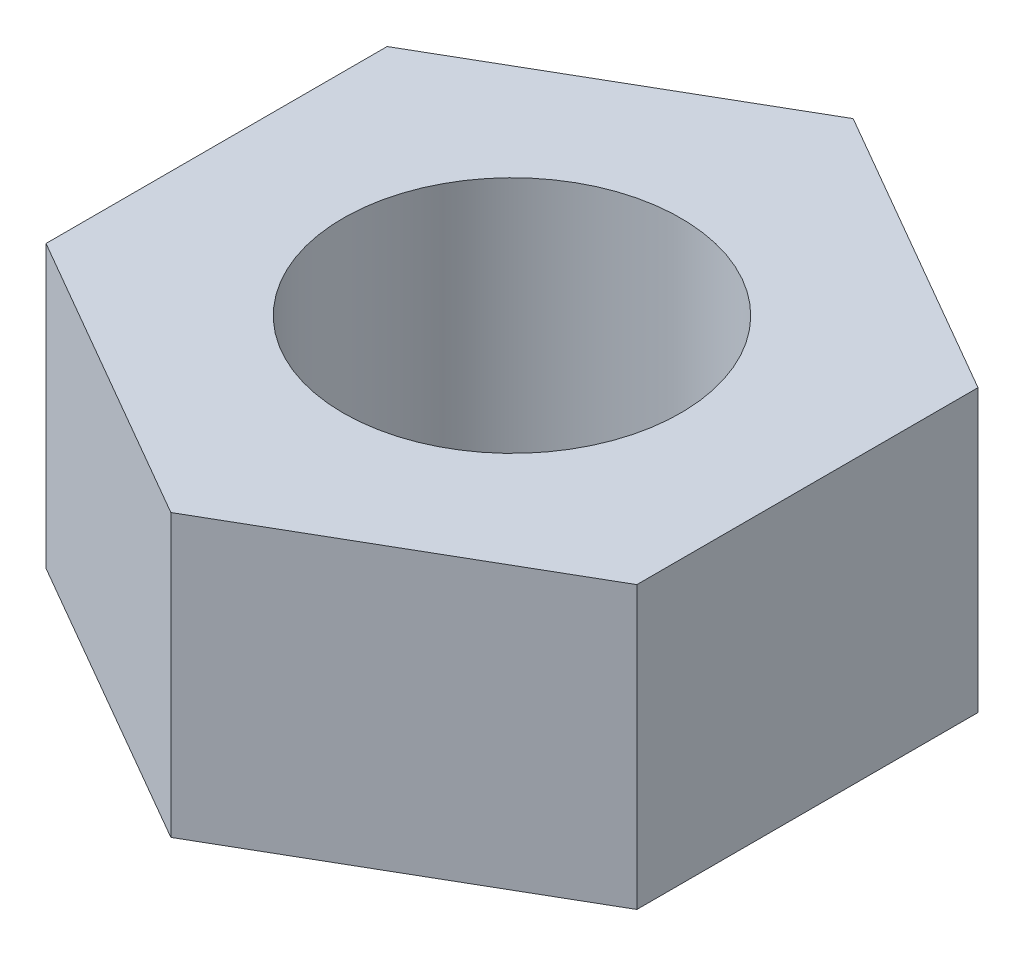
SolidWorks part; units mm, degrees
ref_plane "前视基准面" through (0, 0, 0) normal (0, 0, 1) x (1, 0, 0)
ref_plane "上视基准面" through (0, 0, 0) normal (0, 1, 0) x (1, 0, 0)
ref_plane "右视基准面" through (0, 0, 0) normal (1, 0, 0) x (0, 0, -1)
sketch "草图1" plane through (0, 0, 0) normal (0, 1, 0) x (1, 0, 0)
  line L0 (0, 0.866) -> (0, 20.5922) construction
  line L1 (0, 12.1244) -> (-10.5, 6.0622)
  line L2 (-10.5, 6.0622) -> (-10.5, -6.0622)
  line L3 (-10.5, -6.0622) -> (0, -12.1244)
  line L4 (0, -12.1244) -> (10.5, -6.0622)
  line L5 (10.5, -6.0622) -> (10.5, 6.0622)
  line L6 (10.5, 6.0622) -> (0, 12.1244)
  circle A0 centre (0, 0) radius 10.5 construction
  dimension "D1" = 21
extrude "凸台-拉伸1" add sketch "草图1" along normal blind 10
hole_wizard "M14 螺纹孔1" positions "草图3" profile "草图2" tap size "M14" standard "ISO" end condition through all
sketch "草图3" plane through (0, 10, 0) normal (0, 1, 0) x (1, 0, 0)
  point P0 (0, 0)
sketch "草图2" plane through (0, 10, 0) normal (1, 0, 0) x (0, 0, 1)
  line L0 (0, 0) -> (0, 10)
  line L1 (0, 10) -> (6, 10)
  line L2 (6, 10) -> (6, 0)
  line L5 (6, 0) -> (0, 0)
  line L11 (0, -6.35) -> (0, 107.95) construction
  dimension "通孔螺纹孔钻头直径" = 12
  dimension "通孔螺纹孔钻头深度" = 10
cosmetic thread "孔螺蚊线1" parameters "D2"=14
